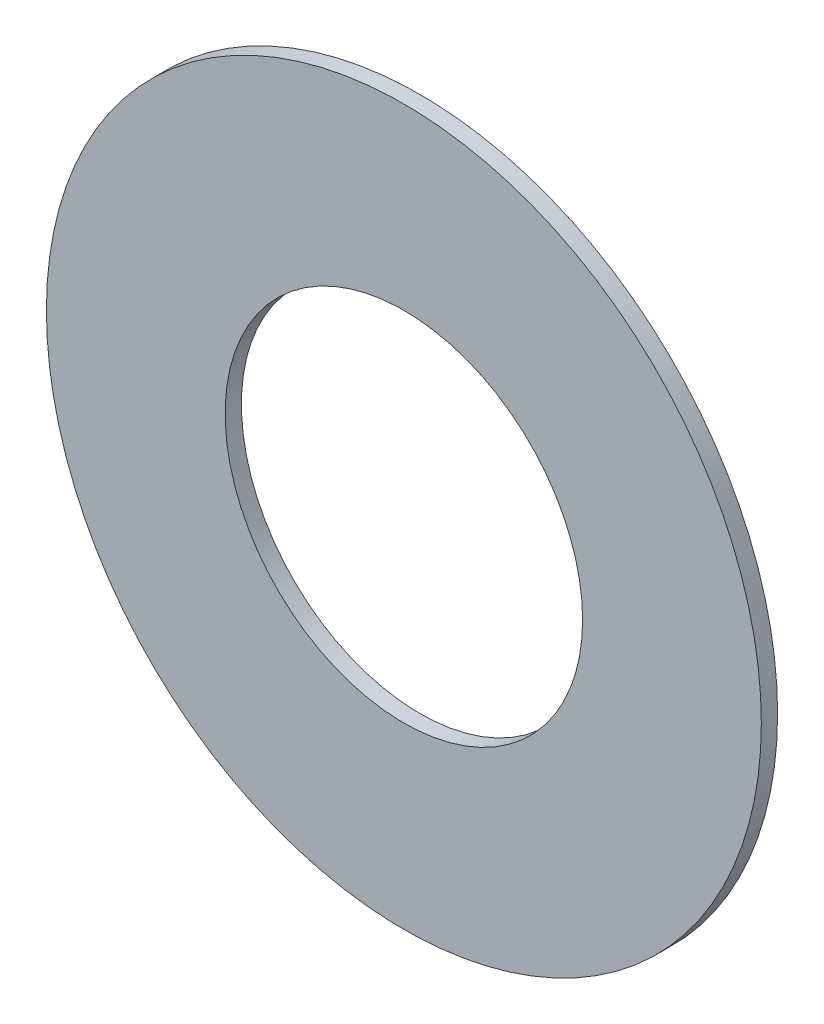
SolidWorks part; units mm, degrees
ref_plane "Front Plane" through (0, 0, 0) normal (0, 0, 1) x (1, 0, 0)
ref_plane "Top Plane" through (0, 0, 0) normal (0, 1, 0) x (1, 0, 0)
ref_plane "Right Plane" through (0, 0, 0) normal (1, 0, 0) x (0, 0, -1)
sketch "Sketch1" plane through (0, 0, 0) normal (0, 0, 1) x (1, 0, 0)
  circle A0 centre (-2.717, 0.5838) radius 55
  circle A1 centre (-2.717, 0.5838) radius 110
extrude "Boss-Extrude3" add sketch "Sketch1" along normal blind 5 contours A0 | A1
